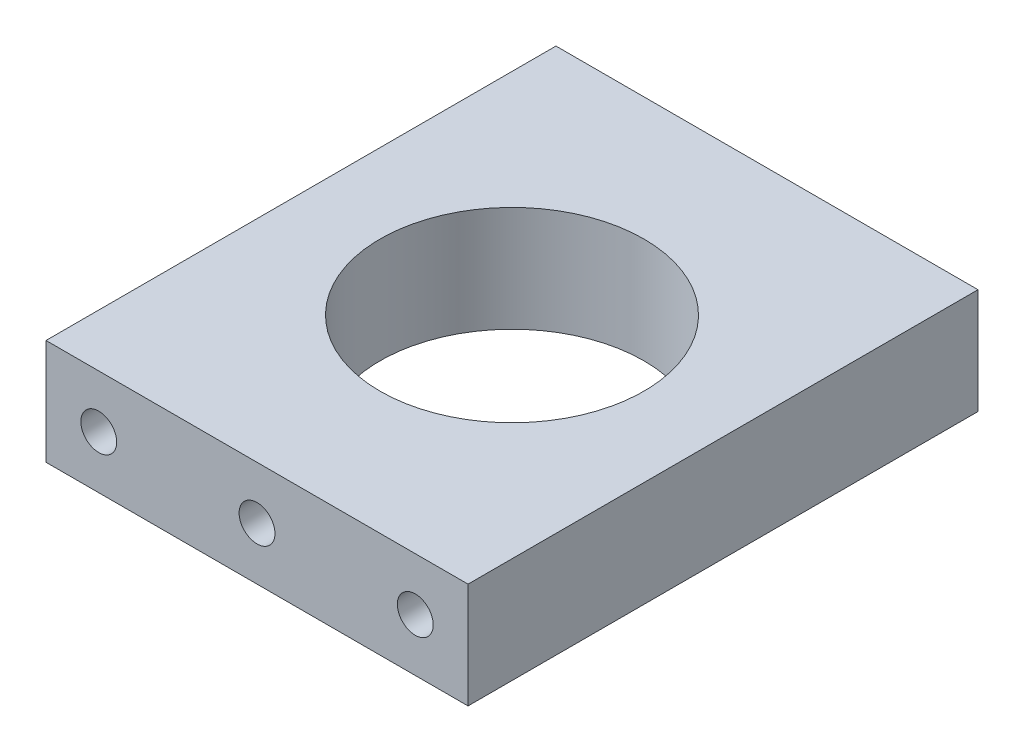
SolidWorks part; units mm, degrees
material "普通碳钢"
ref_plane "前视基准面" through (0, 0, 0) normal (0, 0, 1) x (1, 0, 0)
ref_plane "上视基准面" through (0, 0, 0) normal (0, 1, 0) x (1, 0, 0)
ref_plane "右视基准面" through (0, 0, 0) normal (1, 0, 0) x (0, 0, -1)
sketch "草图1" plane through (0, 0, 0) normal (0, 1, 0) x (1, 0, 0)
  line L1 (-60, -72.5) -> (60, -72.5)
  line L2 (-60, -72.5) -> (-60, 72.5)
  line L3 (-60, 72.5) -> (60, 72.5)
  line L4 (60, -72.5) -> (60, 72.5)
  line L5 (-60, -72.5) -> (60, 72.5) construction
  line L6 (-60, 72.5) -> (60, -72.5) construction
  circle A0 centre (0, 0) radius 37.5
  point P0 (0, 0)
  dimension "D1" = 75
  dimension "D2" = 120
  dimension "D3" = 145
extrude "凸台-拉伸1" add sketch "草图1" along normal blind 30
hole_wizard "M10 螺纹孔1" positions "草图2" profile "草图3" tap size "M10" standard "GB"
sketch "草图2" plane through (0, 0, 0) normal (0, -1, 0) x (-1, 0, 0)
  line L0 (-60, -72.5) -> (-60, 72.5) construction
  line L1 (60, -72.5) -> (-60, -72.5) construction
  point P0 (-32.8805, -32.8805)
  point P2 (-44.9156, -12.0351)
  point P4 (-44.9156, 12.0351)
  point P6 (-32.8805, 32.8805)
  point P8 (32.8805, 32.8805)
  point P10 (44.9156, 12.0351)
  point P12 (44.9156, -12.0351)
  point P14 (32.8805, -32.8805)
  dimension "D1" = 15.0844
  dimension "D2" = 27.1195
  dimension "D3" = 92.8805
  dimension "D4" = 104.9156
  dimension "D5" = 39.6195
  dimension "D6" = 60.4649
  dimension "D7" = 84.5351
  dimension "D8" = 105.3805
sketch "草图3" plane through (32.8805, 0, 32.8805) normal (1, 0, 0) x (0, 0, -1)
  line L0 (0, 0) -> (0, 27.0537)
  line L1 (0, 27.0537) -> (4.25, 24.5)
  line L2 (4.25, 24.5) -> (4.25, 0)
  line L5 (4.25, 0) -> (0, 0)
  line L10 (0, 27.0537) -> (-4.25, 24.5) construction
  line L11 (0, -6.35) -> (0, 107.95) construction
  dimension "螺纹孔钻头直径" = 8.5
  dimension "螺纹孔钻头深度" = 24.5
  dimension "导头角度" = 118
cosmetic thread "孔螺蚊线1" parameters "D1"=20, "D2"=10
cosmetic thread "孔螺蚊线2" parameters "D1"=20, "D2"=10
cosmetic thread "孔螺蚊线3" parameters "D1"=20, "D2"=10
cosmetic thread "孔螺蚊线4" parameters "D1"=20, "D2"=10
cosmetic thread "孔螺蚊线5" parameters "D1"=20, "D2"=10
cosmetic thread "孔螺蚊线6" parameters "D1"=20, "D2"=10
cosmetic thread "孔螺蚊线7" parameters "D1"=20, "D2"=10
cosmetic thread "孔螺蚊线8" parameters "D1"=20, "D2"=10
hole_wizard "M12 螺纹孔1" positions "草图6" profile "草图5" tap size "M12" standard "GB"
sketch "草图6" plane through (0, 0, -72.5) normal (0, 0, -1) x (-1, 0, 0)
  line L0 (60, 15) -> (45, 15) construction
  line L1 (60, 30) -> (60, 0) construction
  line L2 (45, 15) -> (0, 15) construction
  line L3 (0, 15) -> (-45, 15) construction
  line L8 (-45, 15) -> (-60, 15) construction
  line L9 (-60, 30) -> (-60, 0) construction
  point P0 (45, 15)
  point P2 (0, 15)
  point P4 (-45, 15)
  dimension "D1" = 15
sketch "草图5" plane through (-45, 15, -72.5) normal (1, 0, 0) x (0, 1, 0)
  line L0 (0, 0) -> (0, 32.3144)
  line L1 (0, 32.3144) -> (5.1, 29.25)
  line L2 (5.1, 29.25) -> (5.1, 0)
  line L5 (5.1, 0) -> (0, 0)
  line L10 (0, 32.3144) -> (-5.1, 29.25) construction
  line L11 (0, -6.35) -> (0, 107.95) construction
  dimension "螺纹孔钻头直径" = 10.2
  dimension "螺纹孔钻头深度" = 29.25
  dimension "导头角度" = 118
cosmetic thread "孔螺蚊线9" parameters "D1"=24, "D2"=12
cosmetic thread "孔螺蚊线10" parameters "D1"=24, "D2"=12
cosmetic thread "孔螺蚊线11" parameters "D1"=24, "D2"=12
mirror "镜向1" about plane through (0, 0, 0) normal (0, 0, 1) of "M12 螺纹孔1"
